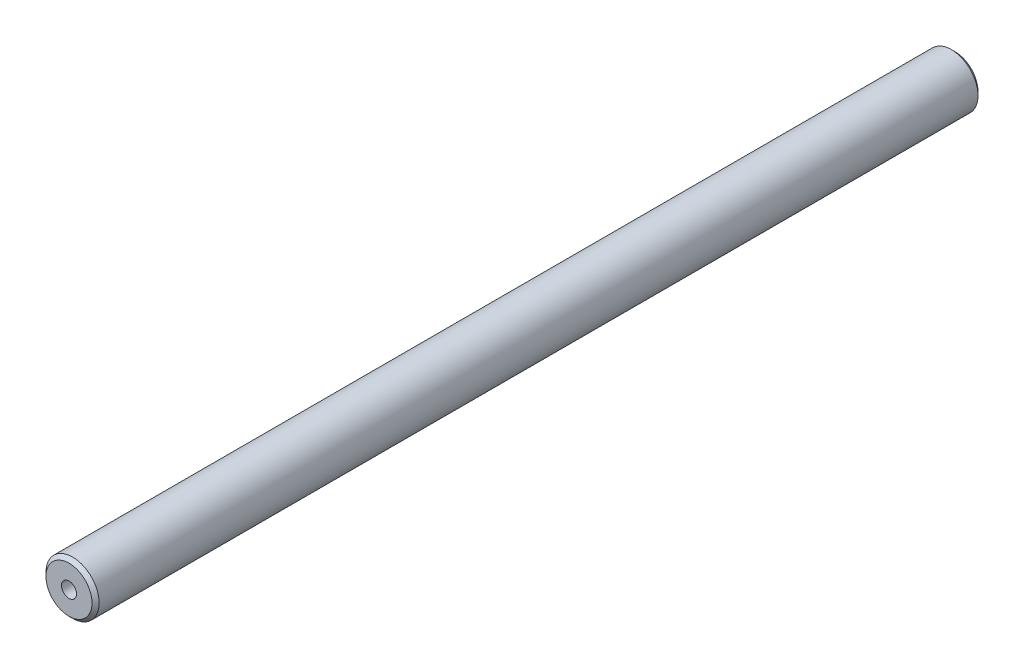
from build123d import *

# Parameters (mm, degrees)
SKETCH1_R              = 15
BOSS_EXTRUDE1_DEPTH    = 500
CHAMFER1_SIZE          = 2
M10_TAPPED_HOLE1_D     = 8.5
M10_TAPPED_HOLE1_DEPTH = 24.5
M10_TAPPED_HOLE1_TIP   = 2.553657631


with BuildPart() as part:
    # Sketch1 → Boss-Extrude1 (new body)
    with BuildSketch(Plane.XY):
        Circle(SKETCH1_R)
    extrude(amount=BOSS_EXTRUDE1_DEPTH)

    # Chamfer1
    chamfer1_edges = [part.edges().sort_by_distance(p)[0] for p in [
        (-15, 0, 0),
        (-15, 0, 500),
    ]]
    chamfer(chamfer1_edges, length=CHAMFER1_SIZE)

    # M10 Tapped Hole1
    with Locations(Plane.XY.offset(500)):
        with Locations((0, 0)):
            Hole(M10_TAPPED_HOLE1_D / 2, depth=M10_TAPPED_HOLE1_DEPTH)
            with Locations((0, 0, -(M10_TAPPED_HOLE1_DEPTH + M10_TAPPED_HOLE1_TIP / 2))):  # 118° drill point
                Cone(0, M10_TAPPED_HOLE1_D / 2, M10_TAPPED_HOLE1_TIP, mode=Mode.SUBTRACT)


solid = part.part
